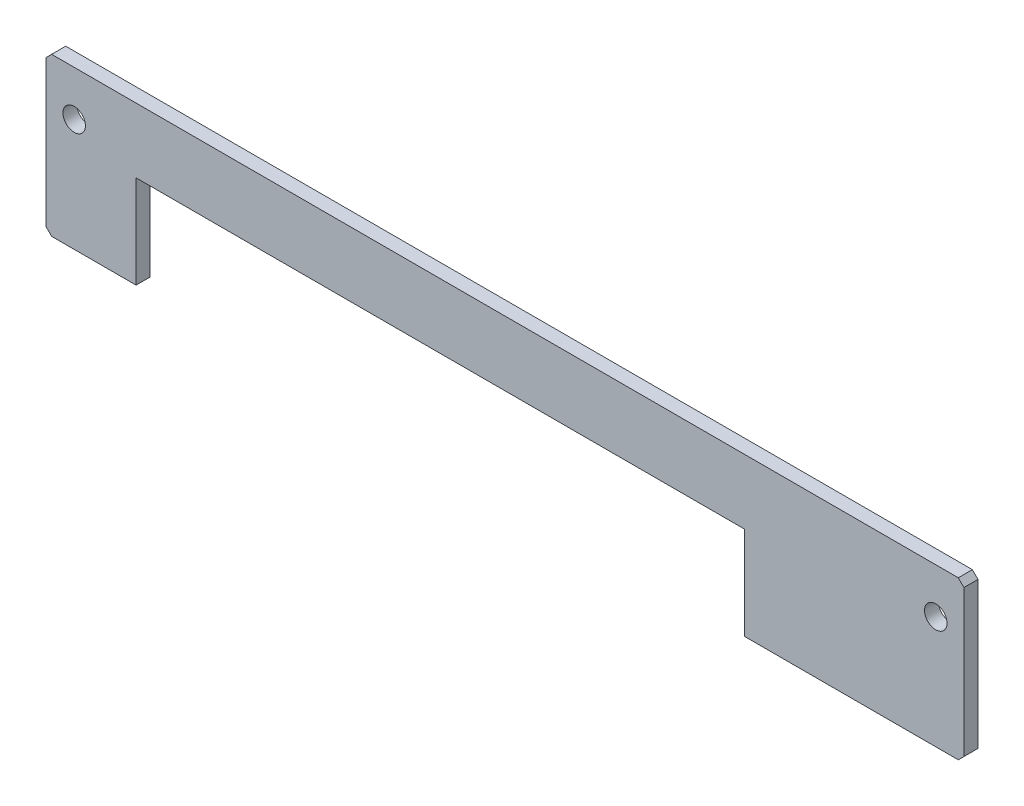
SolidWorks part; units mm, degrees
ref_plane "前视基准面" through (0, 0, 0) normal (0, 0, 1) x (1, 0, 0)
ref_plane "上视基准面" through (0, 0, 0) normal (0, 1, 0) x (1, 0, 0)
ref_plane "右视基准面" through (0, 0, 0) normal (1, 0, 0) x (0, 0, -1)
sketch "草图1" plane through (0, 0, 0) normal (0, 0, 1) x (1, 0, 0)
  line L0 (160, -280) -> (0, -280)
  line L5 (160, -115) -> (1240, -115)
  line L6 (1240, -115) -> (1240, -280)
  line L8 (1630, 0) -> (1630, -280)
  line L9 (1630, -280) -> (1240, -280)
  line L10 (0, 0) -> (0, -280)
  line L13 (160, -115) -> (160, -280)
  line L14 (1630, 0) -> (0, 0)
  point P0 (0, 0)
  point P2 (0, 0)
  point P4 (1044.3195, 251.0586)
  point P11 (623.9859, 264.3808)
  dimension "D1" = 1080
  dimension "D2" = 160
  dimension "D3" = 390
  dimension "D4" = 280
  dimension "D5" = 165
extrude "凸台-拉伸1" add sketch "草图1" along normal blind 25
chamfer "倒角1" distance 10 angle 45 4 edges at (0, 0, 12.5) (0, -280, 12.5) (1630, -280, 12.5) (1630, 0, 12.5)
sketch "草图2" plane through (0, 0, 25) normal (0, 0, 1) x (1, 0, 0)
  line L0 (0, -10) -> (0, -270) construction
  line L1 (1620, 0) -> (10, 0) construction
  line L2 (1630, -270) -> (1630, -10) construction
  circle A0 centre (50, -80) radius 20
  circle A1 centre (1580, -80) radius 20
  dimension "D3" = 40
  dimension "D4" = 40
  dimension "D1" = 50
  dimension "D2" = 80
  dimension "D5" = 50
  dimension "D6" = 80
extrude "切除-拉伸1" cut sketch "草图2" against normal through all both and the other way through all
